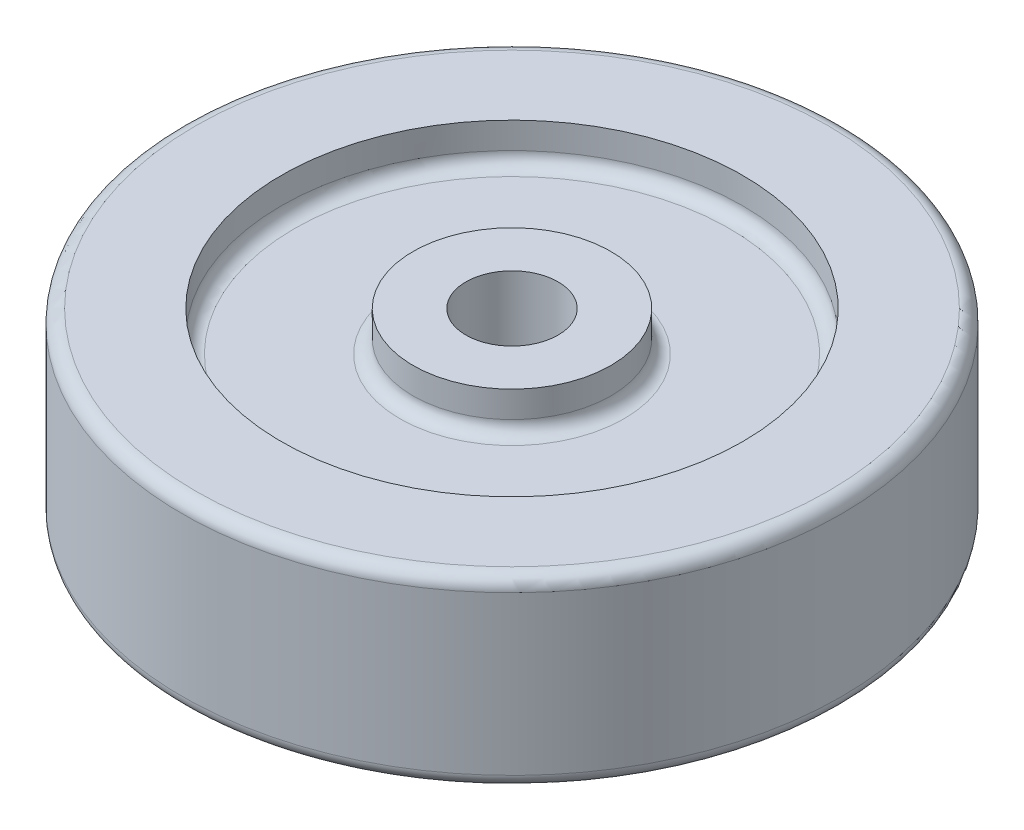
from build123d import *

# Parameters (mm, degrees)
FILLET2_R = 2
FILLET4_R = 2


with BuildPart() as part:
    # Sketch1 → Revolve1 (revolve)
    with BuildSketch(Plane.XY):
        Polygon((15, 8), (35, 8), (35, 14), (50, 14), (50, -14), (35, -14), (35, -8), (15, -8), (15, -14), (7, -14), (7, 14), (15, 14), align=None)
    revolve(axis=Axis((0, -499.994958486, 0), (0, 1, 0)))

    # Fillet2
    fillet2_edges = [part.edges().sort_by_distance(p)[0] for p in [
        (-15, 8, 0),
        (-35, 8, 0),
        (-50, 14, 0),
    ]]
    fillet(fillet2_edges, radius=FILLET2_R)

    # Fillet4
    fillet4_edges = [part.edges().sort_by_distance(p)[0] for p in [
        (-50, -14, 0),
        (-35, -8, 0),
        (-15, -8, 0),
    ]]
    fillet(fillet4_edges, radius=FILLET4_R)


solid = part.part
